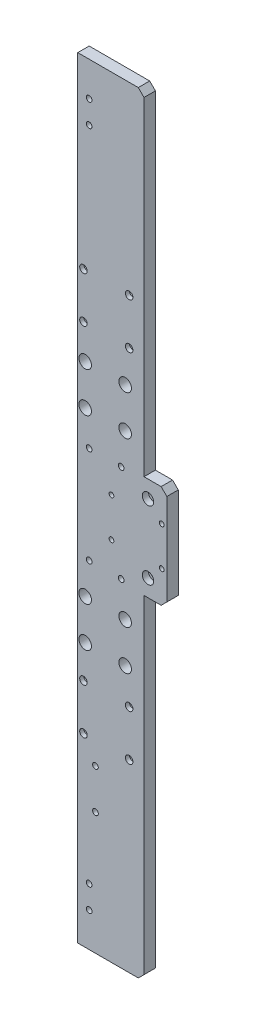
from build123d import *

# Parameters (mm, degrees)
SKETCH_1_W                     = 108
SKETCH_1_H                     = 675
EXTRUDE_1_DEPTH                = 10
HOLE_WIZARD_M6_1_D             = 5
HOLE_WIZARD_M6_1_2_D           = 6.6
HOLE_WIZARD_M6_1_2_CBORE_D     = 11
HOLE_WIZARD_M6_1_2_CBORE_DEPTH = 6.4
HOLE_WIZARD_M5_1_D             = 4.2
HOLE_WIZARD_M5_1_DEPTH         = 14
HOLE_WIZARD_M5_1_TIP           = 1.2618073
HOLE_WIZARD_M6_2_D             = 5
HOLE_WIZARD_M6_2_DEPTH         = 17
HOLE_WIZARD_M6_2_TIP           = 1.502151548
HOLE_WIZARD_M5_1_2_D           = 5.5
HOLE_WIZARD_M5_1_2_DEPTH       = 14
HOLE_WIZARD_M5_1_2_CBORE_D     = 10
HOLE_WIZARD_M5_1_2_CBORE_DEPTH = 5.4
HOLE_WIZARD_M5_1_2_TIP         = 1.652366702
HOLE_WIZARD_M6_3_D             = 5
HOLE_WIZARD_M6_3_DEPTH         = 17
HOLE_WIZARD_M6_3_TIP           = 1.502151548
SKETCH_14_R                    = 5.5
CUT_EXTRUDE_1_DEPTH            = 60
SKETCH_15_R                    = 2.5
SKETCH_15_W                    = 30
SKETCH_15_H                    = 90
SKETCH_15_R_2                  = 5
CUT_EXTRUDE_2_DEPTH            = 684.658540501
CHAMFER_1_SIZE                 = 5
HOLE_WIZARD_M6_4_D             = 5


with BuildPart() as part:
    # 草图1 → 凸台-拉伸1 (new body)
    with BuildSketch(Plane.XY):
        with Locations((54, 337.5)):
            Rectangle(SKETCH_1_W, SKETCH_1_H)
    extrude(amount=EXTRUDE_1_DEPTH)

    # Hole Wizard M6 _1 (through all)
    with Locations(Plane.XY.offset(10)):
        with Locations((10, 645), (10, 625), (10, 50), (10, 30)):
            Hole(HOLE_WIZARD_M6_1_D / 2)

    # Hole Wizard M6 _1 2 (through all)
    with Locations(Plane(origin=(0, 0, 0), x_dir=(-1, 0, 0), z_dir=(0, 0, -1))):
        with Locations((-45, 513.5), (-5, 513.5), (-45, 473.5), (-5, 473.5), (-5, 201.5), (-45, 201.5), (-5, 161.5), (-45, 161.5)):
            CounterBoreHole(HOLE_WIZARD_M6_1_2_D / 2, HOLE_WIZARD_M6_1_2_CBORE_D / 2, HOLE_WIZARD_M6_1_2_CBORE_DEPTH)

    # Hole Wizard M5 _1
    with Locations(Plane.XY.offset(10)):
        with Locations((29.5, 354.5), (73.5, 354.5), (29.5, 320.5), (73.5, 320.5)):
            Hole(HOLE_WIZARD_M5_1_D / 2, depth=HOLE_WIZARD_M5_1_DEPTH)
            with Locations((0, 0, -(HOLE_WIZARD_M5_1_DEPTH + HOLE_WIZARD_M5_1_TIP / 2))):  # 118° drill point
                Cone(0, HOLE_WIZARD_M5_1_D / 2, HOLE_WIZARD_M5_1_TIP, mode=Mode.SUBTRACT)

    # M6 螺纹孔2
    with Locations(Plane.XY.offset(10)):
        with Locations((97.5, 431.5), (97.5, 396.5)):
            Hole(HOLE_WIZARD_M6_2_D / 2, depth=HOLE_WIZARD_M6_2_DEPTH)
            with Locations((0, 0, -(HOLE_WIZARD_M6_2_DEPTH + HOLE_WIZARD_M6_2_TIP / 2))):  # 118° drill point
                Cone(0, HOLE_WIZARD_M6_2_D / 2, HOLE_WIZARD_M6_2_TIP, mode=Mode.SUBTRACT)

    # Hole Wizard M5 _1 2
    with Locations(Plane.XY.offset(10)):
        with Locations((61.5, 367.5), (91.5, 367.5), (61.5, 307.5), (91.5, 307.5)):
            CounterBoreHole(HOLE_WIZARD_M5_1_2_D / 2, HOLE_WIZARD_M5_1_2_CBORE_D / 2, HOLE_WIZARD_M5_1_2_CBORE_DEPTH, depth=HOLE_WIZARD_M5_1_2_DEPTH)
            with Locations((0, 0, -(HOLE_WIZARD_M5_1_2_DEPTH + HOLE_WIZARD_M5_1_2_TIP / 2))):  # 118° drill point
                Cone(0, HOLE_WIZARD_M5_1_2_D / 2, HOLE_WIZARD_M5_1_2_TIP, mode=Mode.SUBTRACT)

    # M6 螺纹孔3
    with Locations(Plane(origin=(0, 0, 0), x_dir=(-1, 0, 0), z_dir=(0, 0, -1))):
        with Locations((-38, 380), (-10, 380), (-38, 295), (-10, 295)):
            Hole(HOLE_WIZARD_M6_3_D / 2, depth=HOLE_WIZARD_M6_3_DEPTH)
            with Locations((0, 0, -(HOLE_WIZARD_M6_3_DEPTH + HOLE_WIZARD_M6_3_TIP / 2))):  # 118° drill point
                Cone(0, HOLE_WIZARD_M6_3_D / 2, HOLE_WIZARD_M6_3_TIP, mode=Mode.SUBTRACT)

    # 草图14 → 切除-拉伸1 (cut)
    with BuildSketch(Plane.XY.offset(10)):
        with Locations((41.5, 444)):
            Circle(SKETCH_14_R)
        with Locations((6.5, 444)):
            Circle(SKETCH_14_R)
        with Locations((41.5, 409)):
            Circle(SKETCH_14_R)
        with Locations((6.5, 409)):
            Circle(SKETCH_14_R)
        with Locations((41.5, 266)):
            Circle(SKETCH_14_R)
        with Locations((41.5, 231)):
            Circle(SKETCH_14_R)
        with Locations((6.5, 231)):
            Circle(SKETCH_14_R)
        with Locations((6.5, 266)):
            Circle(SKETCH_14_R)
    extrude(amount=-CUT_EXTRUDE_1_DEPTH, mode=Mode.SUBTRACT)

    # 草图15 → 切除-拉伸2 (cut, through all)
    # profile 1 of 5: a face of its own
    with BuildSketch(Plane.XY.offset(10)):
        Polygon((108, 382.5), (108, 675), (58, 675), (58, 382.5), (78, 382.5), align=None)
        with Locations((97.5, 396.5)):
            Circle(SKETCH_15_R, mode=Mode.SUBTRACT)
        with Locations((97.5, 431.5)):
            Circle(SKETCH_15_R, mode=Mode.SUBTRACT)
    # profile 2 of 5: a face of its own
    with BuildSketch(Plane.XY.offset(10)):
        with Locations((93, 337.5)):
            Rectangle(SKETCH_15_W, SKETCH_15_H)
        with Locations((91.5, 307.5)):
            Circle(SKETCH_15_R_2, mode=Mode.SUBTRACT)
        with Locations((91.5, 367.5)):
            Circle(SKETCH_15_R_2, mode=Mode.SUBTRACT)
    # profile 3 of 5: a face of its own
    with BuildSketch(Plane.XY.offset(10)):
        Polygon((108, 0), (108, 292.5), (78, 292.5), (58, 292.5), (58, 0), align=None)
    # profile 4 of 5: a face of its own
    with BuildSketch(Plane.XY.offset(10)):
        with Locations((91.5, 367.5)):
            Circle(SKETCH_15_R_2)
    # profile 5 of 5: a face of its own
    with BuildSketch(Plane.XY.offset(10)):
        with Locations((91.5, 307.5)):
            Circle(SKETCH_15_R_2)
    extrude(amount=-CUT_EXTRUDE_2_DEPTH, mode=Mode.SUBTRACT)

    # 倒角1
    chamfer_1_edges = [part.edges().sort_by_distance(p)[0] for p in [
        (58, 675, 5),
        (58, 0, 5),
        (78, 292.5, 5),
        (78, 382.5, 5),
    ]]
    chamfer(chamfer_1_edges, length=CHAMFER_1_SIZE)

    # M6 螺纹孔4 (through all)
    with Locations(Plane.XY.offset(10)):
        with Locations((15.5, 142), (15.5, 107)):
            Hole(HOLE_WIZARD_M6_4_D / 2)


solid = part.part
